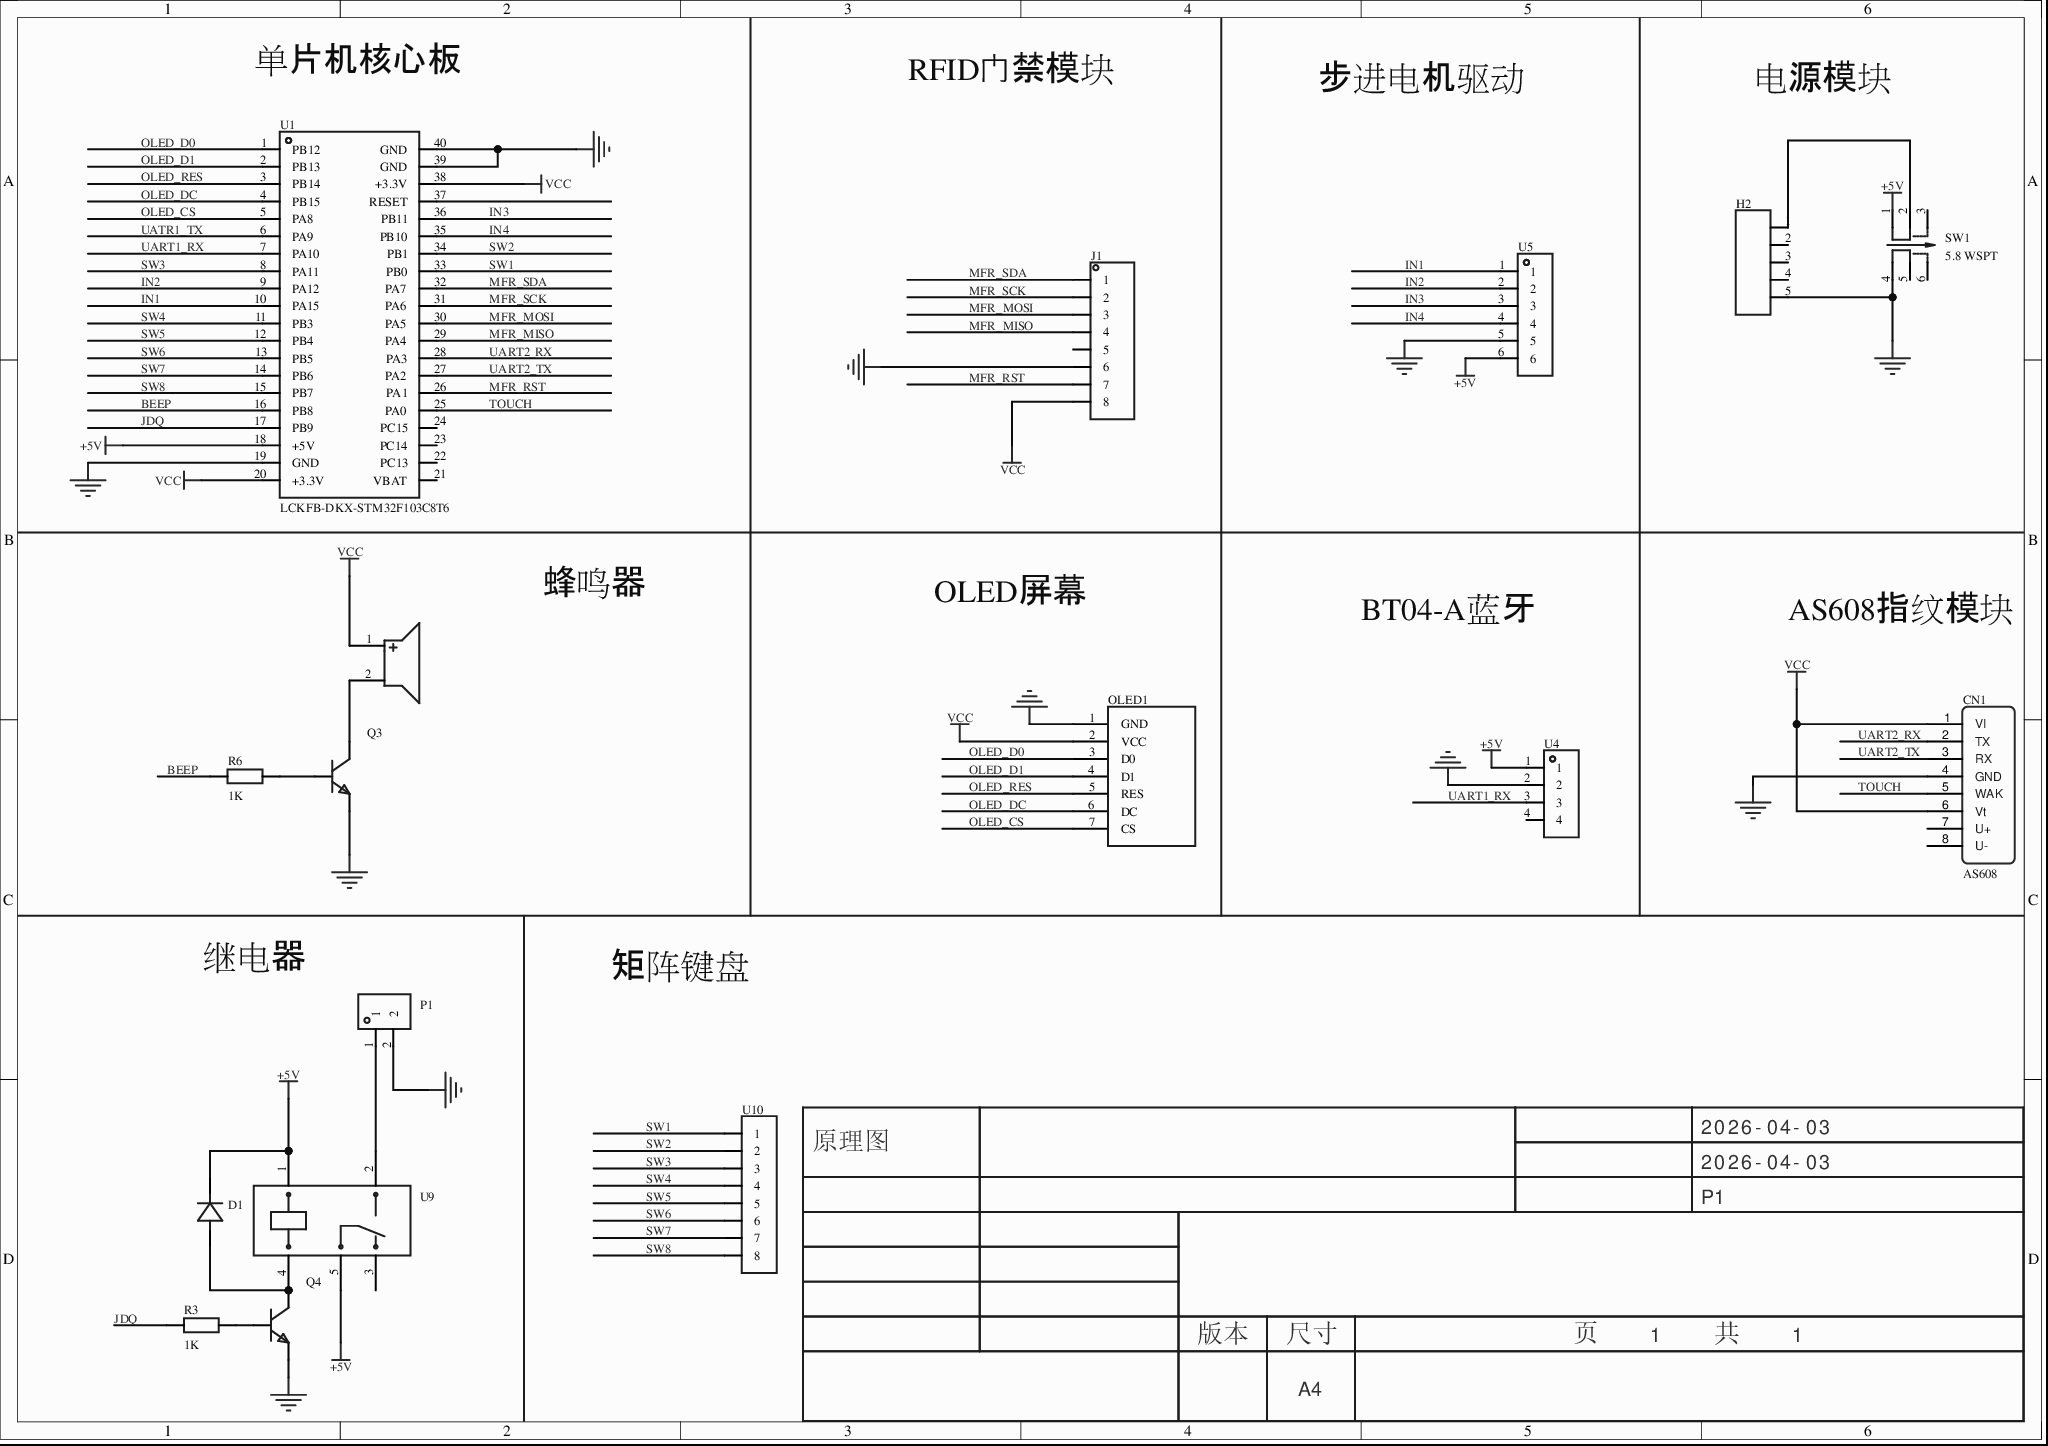
[diagram p0: MISC51826-3.schdoc]
# Altium project MISC51826-2.PrjPcb
1 sheet, 17 parts. Net scope: global (net labels, ports and power ports of the same name join across sheets).
Board file: MISC51826.pcbdoc

## Sheet MISC51826-3.schdoc
size 297 x 209 mm; Version: V1.0; @Project Name: MISC51826; @Update Date: 2026-04-03; @Create Date: 2026-04-03; @Board Name: MISC51826; @Create Time: 23:26:07; @Page Count: 1; @Page No: 1; @Schematic Name: MISC51826; @Update Time: 23:26:07; Size: A4

### Parts
BUZZER1  2.7kHz  [BUZ-TH_BD9.0-P4.00-D0.6-FD]  (value not drawn)
CN1  AS608  [AS608]
D1  (no value)  [DO_1N4007]
H2  (no value)  [HDR-TH_5P-P2.54-V-F]
J1  (no value)  [HDR-TH_8P-P2.54-V-M]
OLED1  (no value)  [0.96OLED]
P1  WAFER-XH254Z-2A  [CONN-TH_2P-P2.50_XH-2A_3045048]  (value not drawn)
Q3  (no value)  [S8050_TO_92]
Q4  (no value)  [S8050_TO_92]
R3  1K  [Res_1/8W]
R6  1K  [Res_1/8W]
SW1  5.8 WSPT  [SW-TH_6P-L5.8-W5.8-P2.00-LS4.5-TL_K8-5851E-L1]
U1  LCKFB-DKX-STM32F103C8T6  [CONN-TH_L53.3-W22.9_STM32F103C8T6-CARD]
U4  (no value)  [HDR-TH_4P-P2.54-V-F]
U5  (no value)  [HDR-TH_6P-P2.54-V-F]
U9  SRD-12VDC-SL-C  [RELAY-TH_SRD-XXVDC-XL-C]  (value not drawn)
U10  (no value)  [HDR-TH_8P-P2.54-V-F-1]

### Nets
+5V: D1.1(K) SW1.1 U1.18(+5V) U4.1 U5.6 U9.1 U9.5
GND: CN1.4(GND) H2.5 J1.6 OLED1.1(GND) P1.2 Q3.1(E) Q4.1(E) SW1.4 U1.19(GND) U1.39(GND) U1.40(GND) U4.2 U5.5
VCC: BUZZER1.1 CN1.1(VI) CN1.6(Vt) J1.8 OLED1.2(VCC) U1.20(+3.3V) U1.38(+3.3V)
BEEP: R6.1 U1.16(PB8)
IN1: U1.10(PA15) U5.1
IN2: U1.9(PA12) U5.2
IN3: U1.36(PB11) U5.3
IN4: U1.35(PB10) U5.4
JDQ: R3.1 U1.17(PB9)
MFR_MISO: J1.4 U1.29(PA4)
MFR_MOSI: J1.3 U1.30(PA5)
MFR_RST: J1.7 U1.26(PA1)
MFR_SCK: J1.2 U1.31(PA6)
MFR_SDA: J1.1 U1.32(PA7)
OLED_CS: OLED1.7(CS) U1.5(PA8)
OLED_D0: OLED1.3(D0) U1.1(PB12)
OLED_D1: OLED1.4(D1) U1.2(PB13)
OLED_DC: OLED1.6(DC) U1.4(PB15)
OLED_RES: OLED1.5(RES) U1.3(PB14)
SW1: U1.33(PB0) U10.1
SW2: U1.34(PB1) U10.2
SW3: U1.8(PA11) U10.3
SW4: U1.11(PB3) U10.4
SW5: U1.12(PB4) U10.5
SW6: U1.13(PB5) U10.6
SW7: U1.14(PB6) U10.7
SW8: U1.15(PB7) U10.8
TOUCH: CN1.5(WAK) U1.25(PA0)
UART1_RX: U1.7(PA10) U4.3
UART2_RX: CN1.2(TX) U1.28(PA3)
UART2_TX: CN1.3(RX) U1.27(PA2)
UATR1_TX: U1.6(PA9)
NetBUZZER1_2: BUZZER1.2 Q3.3(C)
NetD1_2: D1.2(A) Q4.3(C) U9.4
NetH2_1: H2.1 SW1.2
NetP1_1: P1.1 U9.2
NetQ3_2: Q3.2(B) R6.2
NetQ4_2: Q4.2(B) R3.2

Not connected (* = marked no-connect by the designer): CN1 7(U+) 8(U-); H2 2(4) 3 4(2); J1 5; SW1 3 5 6; U1 21(VBAT) 22(PC13) 23(PC14) 24(PC15) 37(RESET); U4 4; U9 3

### Notes on the sheet
- 单片机核心板
- RFID门禁模块
- 步进电机驱动
- 电源模块
- 蜂鸣器
- OLED屏幕
- BT04-A蓝牙
- AS608指纹模块
- 继电器
- 矩阵键盘
- 2026-04-03
- 原理图
- P1
- 版本
- 尺寸
- A4
- 页    1    共    1

### Library data of the parts
BUZZER1 = QMB-09B-03: 驱动方式:无源(外部驱动);构造类型:电磁式;频率:2.7kHz;声压(SPL):85dB;; Manufacturer: 华能; 3D Model: 949096c5110a440bbcfd89e7e6948986; 3D Model Transform: 354.33,354.33,0,90,0,0,0,0,-177.165; Voltage - Supply: 2V~5V; Sound Pressure Level(SPL): 85dB; AddInBom: yes; ModelName: BUZ-TH_D9.0-H5.5-P4.0; Symbol: QMB-09B-03; Device: QMB-09B-03; LCSC Part Name: 无源蜂鸣器QMB-09B-03; Supplier Part: C96256; Manufacturer Part: QMB-09B-03; Supplier Footprint: 插件,D=9mm; JLCPCB Part Class: 扩展库; Datasheet: https://atta.szlcsc.com/upload/public/pdf/source/20210401/C96256_958B17753B5AD7CBFBCFFC7C095B4484.pdf; Supplier: LCSC; Driver Circuitry: 无源(外部驱动); Technology: 电磁式; Value: 2.7kHz; Diameter(φD): 9mm; Height: 5.7mm; ConvertToPcb: yes; FootprintName: BUZ-TH_BD9.0-P4.00-D0.6-FD
CN1 = AS608: Manufacturer: lengyuefeng; 3DModel: CONN-SMD_HC-1.25-8PWT; _: 3; AddInBom: yes; Symbol: AS608; Device: AS608; ConvertToPcb: yes; FootprintName: AS608; Supplier: lengyuefeng
D1 = D_1N4007A: 3D Model: 6de1e9b71a0d4751b4e9df530304c1a3; 3D Model Transform: 373.9,94.4,232.29,0,0,0,0,0,-140; AddInBom: yes; ModelName: DO-41_D2.4-L4.7-P8.70; Symbol: D_1N4007; Device: D_1N4007A; Supplier Footprint: DO-41; ConvertToPcb: yes; FootprintName: DO_1N4007
H2 = HDR-F_2.54_1x5P: Symbol: Header-Female-2.54_1x5; 3D Model: f49cb6116a3d45e5a64915bf3e00773f; 3D Model Transform: 519.684,98.464,0,0,0,0,0,0,-124.016; ConvertToPcb: yes; Device: HDR-F_2.54_1x5P; Supplier Part: C50950; Supplier Footprint: 插件; AddInBom: yes; FootprintName: HDR-TH_5P-P2.54-V-F; ModelName: HDR-TH_5P-P2.54-V-F
J1 = HDR-M_2.54_1x8P: Symbol: Header-Male-2.54_1x8; 3D Model: f5b96e27511e49e38545e53df2320202; 3D Model Transform: 807.87244,98.425,0,0,0,0,0,0,-118.11; ConvertToPcb: yes; Device: HDR-M_2.54_1x8P; Supplier Part: C124381; Supplier Footprint: 插件; AddInBom: yes; FootprintName: HDR-TH_8P-P2.54-V-M; ModelName: HDR-TH_8P-P2.54-V-M
OLED1 = 0.96OLED: _: 3; AddInBom: yes; Symbol: 0.96OLED; Device: 0.96OLED; ConvertToPcb: yes; FootprintName: 0.96OLED
P1 = WAFER-XH254Z-2A: 插针结构:1x2P;间距:2.54mm;安装方式:直插;参考系列:XH;总PIN数:2P;排数:1;每排PIN数:2;额定电流:3A;工作温度范围:-25℃~+85℃;; Manufacturer: HANBO(汉博); 3D Model: a03ee9acfa8e4e25b912a99a3551fb92; 3D Model Transform: 295.275,228.7397,0,0,0,0,0,21.654,-133.858; Pins Structure: 1x2P; Pitch: 2.54mm; Reference Series: XH; Number of PINs Per Row: 2; Current Rating (Max): 3A; AddInBom: yes; Symbol: WAFER-XH254Z-2A; Device: WAFER-XH254Z-2A; LCSC Part Name: WAFER-XH254Z-2A; Supplier Part: C7432682; Manufacturer Part: WAFER-XH254Z-2A; Supplier Footprint: 插件,P=2.5mm; JLCPCB Part Class: 扩展库; Datasheet: https://atta.szlcsc.com/upload/public/pdf/source/20230718/3B4FABA5D38EFB02DAF74E7C2B33D98F.pdf; Supplier: LCSC; Mounting Style: 直插; Number of Pins: 2P; Number of Rows: 1; Operating Temperature Range: -25℃~+85℃; ConvertToPcb: yes; FootprintName: CONN-TH_2P-P2.50_XH-2A_3045048; ModelName: CONN-TH_2P-P2.50_XH-2A_3045048
Q3 Q4 = S8050_TO_NPN: 3D Model: aafe8e06f2154e7c93506efd0d6632dd; 3D Model Transform: 180.78,141.44,417.3,0,0,0,0,0,-200; ConvertToPcb: yes; ModelName: TO-92-3_L4.9-W3.7-P1.27-L; Symbol: S8050_TO_NPN; Device: S8050_TO_NPN; Supplier Footprint: TO-92; AddInBom: yes; FootprintName: S8050_TO_92
R3 = Res_AXIAL-1/8W: Symbol: 电阻; Value: 10kΩ; 3D Model: b2b5ae7ae4c642178fe0039925c86a3f; 3D Model Transform: 282.86,66.88,253.09,0,0,0,0,0,-191; ConvertToPcb: yes; ModelName: RES-TH_BD1.8-L3.2-P7.20-D0.4; Device: Res_AXIAL-1/8W; Supplier Footprint: 轴向引线; AddInBom: yes; FootprintName: Res_1/8W
R6 = Res_AXIAL-1/8W: Symbol: 电阻; 3D Model: b2b5ae7ae4c642178fe0039925c86a3f; 3D Model Transform: 282.86,66.88,253.09,0,0,0,0,0,-191; ConvertToPcb: yes; ModelName: RES-TH_BD1.8-L3.2-P7.20-D0.4; Device: Res_AXIAL-1/8W; Value: 1K; Supplier Footprint: 轴向引线; AddInBom: yes; FootprintName: Res_1/8W
SW1 = 5.8 WSPT: 电路结构:双刀双掷;自锁/无锁:无锁;安装方式:直插;触点电流:100mA;额定电压 (AC):-;额定电压 (DC):30V;带灯:不带;作用力:1.8N;机械寿命:5千次;; Manufacturer: SHOU HAN(首韩); 3D Model: b8faad98a5c645e9866333cdaba903c3; 3D Model Transform: 229.1334,228.346,0,0,0,0,0,0,-137.795; Circuit: 双刀双掷; Self Lock / No Lock: 无锁; Actuator Style: 矩形柱塞; Contact Current: 100mA; Voltage Rating (DC): 30V; Insulation Resistance: 100MΩ; Actuator/Cap Color: 蓝色; With Lamp: 不带; Pin Style: PC引脚; Operating Force: 1.8N; Mechanical Life: 5千次; AddInBom: yes; Symbol: 5.8 WSPT; Device: 5.8 WSPT; LCSC Part Name: 按键开关5.8x5.8 无锁平头 180gf; Supplier Part: C5379898; Manufacturer Part: 5.8 WSPT; Supplier Footprint: 插件; JLCPCB Part Class: 扩展库; Datasheet: https://atta.szlcsc.com/upload/public/pdf/source/20230323/C831DDA43A625CDC196CB35781CDAE7F.pdf; Supplier: LCSC; IP Rating: -; Mounting Style: 直插; Voltage Rating (AC): -; Operating Temperature: -10℃~+70℃; ConvertToPcb: yes; FootprintName: SW-TH_6P-L5.8-W5.8-P2.00-LS4.5-TL_K8-5851E-L1; ModelName: SW-TH_6P-L5.8-W5.8-P2.00-LS4.5-TL_K8-5851E-L1
U1 = LCKFB-DKX-STM32F103C8T6: Manufacturer: 立创开发板; AddInBom: yes; Symbol: LCKFB-DKX-STM32F103C8T6; Device: LCKFB-DKX-STM32F103C8T6; LCSC Part Name: 立创·地阔星-STM32F103C8T6开发板; Supplier Part: C22396880; Manufacturer Part: LCKFB-DKX-STM32F103C8T6; Supplier Footprint: -; JLCPCB Part Class: 扩展库; Datasheet: https://atta.szlcsc.com/upload/public/pdf/source/20240801/7EEF69F7480DF7C6DA98696664D658D4.pdf; Supplier: LCSC; ConvertToPcb: yes; FootprintName: CONN-TH_L53.3-W22.9_STM32F103C8T6-CARD
U4 = HDR-F_2.54_1x4P: Symbol: 2.54-1*4P母; 3D Model: d187812051054f85879fcaa51a310d8e; 3D Model Transform: 419.6842,98.464,0,0,0,0,0,0,-118.11; ConvertToPcb: yes; Device: HDR-F_2.54_1x4P; Supplier Part: C2718488; Supplier Footprint: 插件; AddInBom: yes; FootprintName: HDR-TH_4P-P2.54-V-F; ModelName: HDR-TH_4P-P2.54-V-F
U5 = HDR-F_2.54_1x6P: Symbol: Header-Female-2.54_1x6; 3D Model: 0f5bcf94dcda47d085f24cdca1696fe9; 3D Model Transform: 619.684,94.488,0,0,0,0,0,0,-125.984; ConvertToPcb: yes; Device: HDR-F_2.54_1x6P; Supplier Part: C40877; Supplier Footprint: 插件; AddInBom: yes; FootprintName: HDR-TH_6P-P2.54-V-F; ModelName: HDR-TH_6P-P2.54-V-F
U9 = SRD-12VDC-SL-C: 线圈电压:12V;触点形式:一组转换:1C(单刀双掷-转换);触点容量(电阻负载):-;最大切换电压:250V@AC;最大切换电流:15A;; Manufacturer: 松乐; 3D Model: d0eda9b8bf8746d18ae810ab88dc78e7; 3D Model Transform: 755.904,622.4397,0,0,0,0,34.882,0,-118.11; Coil Voltage: 12V; Pin Number: 5; Coil Rated Power: 360mW; Maximum Switching Current: 15A; Coil Type: 无极性-单线圈; Coil Resistance: 400Ω; Contact Resistance: 100mΩ; Operate Time: 10ms; AddInBom: yes; ModelName: RELAY-TH_L19.2-W15.6-H15.8; Symbol: SRD-12VDC-SL-C; Device: SRD-12VDC-SL-C; LCSC Part Name: SRD-12VDC-SL-C; Supplier Part: C30431; Manufacturer Part: SRD-12VDC-SL-C; Supplier Footprint: 插件,15.6x19.2mm; JLCPCB Part Class: 扩展库; Datasheet: https://atta.szlcsc.com/upload/public/pdf/source/20200305/C490149_C96E4098A3B1FFB377D5AD2E40B7C2A8.pdf; Supplier: LCSC; Contact Form: 一组转换:1C(单刀双掷-转换); Contact Rating: -; Maximum Switching Voltage: 250V@AC; Release Time: 10ms; ConvertToPcb: yes; FootprintName: RELAY-TH_SRD-XXVDC-XL-C
U10 = HDR-F_2.54_1x8P: Symbol: Header-Female-2.54_1x8; 3D Model: 0f7e4d9227ef4fa08d5469c22cc70cdb; 3D Model Transform: 799.99844,100,0,0,0,0,0,0,-118.11; AddInBom: yes; ModelName: HDR-F-2.54_1x8; Device: HDR-F_2.54_1x8P; Supplier Part: C27438; Supplier Footprint: 插件; ConvertToPcb: yes; FootprintName: HDR-TH_8P-P2.54-V-F-1